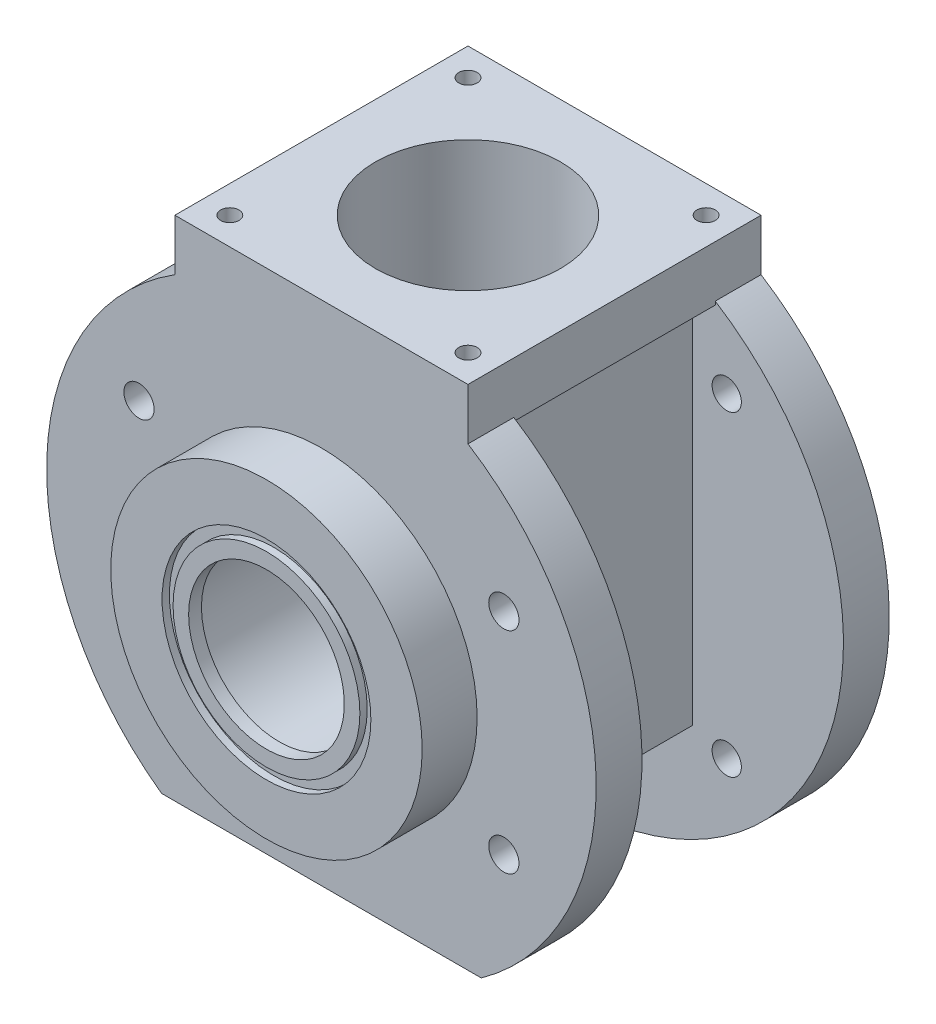
SolidWorks part; units mm, degrees
ref_plane "Front Plane" through (0, 0, 0) normal (0, 0, 1) x (1, 0, 0)
ref_plane "Top Plane" through (0, 0, 0) normal (0, 1, 0) x (1, 0, 0)
ref_plane "Right Plane" through (0, 0, 0) normal (1, 0, 0) x (0, 0, -1)
ref_plane "Plane1" through (0, 0, -520.693) normal (0, 0, -1) x (-1, 0, 0)
sketch "Sketch1" plane through (0, 0, -520.693) normal (0, 0, -1) x (-1, 0, 0)
  line L0 (-441.2306, 361.6297) -> (-601.2306, 361.6297)
  arc A0 (-601.2306, 361.6297) -> (-441.2306, 361.6297) centre (-521.2306, 234.744) ccw
  dimension "D1" = 150
  dimension "D2" = 80
extrude "Boss-Extrude1" add sketch "Sketch1" against normal blind 25
sketch "Sketch2" plane through (0, 0, -495.693) normal (0, 0, 1) x (1, 0, 0)
  line L0 (441.2306, 361.6297) -> (601.2306, 361.6297)
  line L1 (601.2306, 361.6297) -> (601.2306, 154.744)
  line L2 (601.2306, 154.744) -> (441.2306, 154.744)
  line L3 (441.2306, 154.744) -> (441.2306, 361.6297)
  dimension "D1" = 160
  dimension "D2" = 206.8858
extrude "Boss-Extrude2" add sketch "Sketch2" along normal blind 110
sketch "Sketch3" plane through (0, 0, -385.693) normal (0, 0, 1) x (1, 0, 0)
  line L0 (608.5003, 112.744) -> (433.9609, 112.744)
  line L1 (441.2306, 361.6297) -> (601.2306, 361.6297)
  line L2 (441.2306, 361.6297) -> (441.2306, 154.744) construction
  line L3 (441.2306, 154.744) -> (601.2306, 154.744) construction
  arc A0 (601.2306, 361.6297) -> (608.5003, 112.744) centre (521.2306, 234.744) cw
  arc A1 (433.9609, 112.744) -> (441.2306, 361.6297) centre (521.2306, 234.744) cw
  dimension "D1" = 150
  dimension "D2" = 150
  dimension "D3" = 80
  dimension "D4" = 160
  dimension "D5" = 167.2697
  dimension "D6" = 80
extrude "Boss-Extrude3" add sketch "Sketch3" along normal blind 25
sketch "Sketch4" plane through (0, 361.6297, 0) normal (0, 1, 0) x (-1, 0, 0)
  line L0 (-601.2306, -520.693) -> (-601.2306, -360.693)
  line L1 (-601.2306, -360.693) -> (-441.2306, -360.693)
  line L2 (-441.2306, -360.693) -> (-441.2306, -520.693)
  line L3 (-441.2306, -520.693) -> (-601.2306, -520.693)
  line L4 (-441.2306, -495.693) -> (-441.2306, -520.693) construction
  line L5 (-441.2306, -520.693) -> (-601.2306, -520.693) construction
  dimension "D1" = 160
  dimension "D2" = 160
extrude "Boss-Extrude4" add sketch "Sketch4" along normal blind 28.1142
ref_plane "Plane2" through (601.2306, 0, 0) normal (1, 0, 0) x (0, 0, -1)
ref_plane "Plane3" through (588.7306, 0, 0) normal (-1, 0, 0) x (0, -1, 0)
sketch "Sketch6" plane through (588.7306, 0, 0) normal (-1, 0, 0) x (0, -1, 0)
  line L0 (-359.744, -495.693) -> (-154.744, -495.693)
  line L1 (-154.744, -495.693) -> (-154.744, -385.693)
  line L2 (-154.744, -385.693) -> (-359.744, -385.693)
  line L3 (-359.744, -385.693) -> (-359.744, -495.693)
  dimension "D1" = 205
  dimension "D2" = 110
extrude "Cut-Extrude1" cut sketch "Sketch6" against normal up to surface up to plane "Plane2"
ref_plane "Plane4" through (0, 154.744, 0) normal (0, -1, 0) x (1, 0, 0)
ref_plane "Plane5" through (0, 359.744, 0) normal (0, 1, 0) x (1, 0, 0)
sketch "Sketch8" plane through (0, 359.744, 0) normal (0, 1, 0) x (1, 0, 0)
  line L0 (453.7306, 495.693) -> (441.2306, 495.693)
  line L1 (441.2306, 495.693) -> (441.2306, 385.693)
  line L2 (441.2306, 385.693) -> (453.7306, 385.693)
  line L3 (453.7306, 385.693) -> (453.7306, 495.693)
  dimension "D1" = 12.5
  dimension "D2" = 110
extrude "Cut-Extrude2" cut sketch "Sketch8" against normal up to surface up to plane "Plane4"
sketch "Sketch9" plane through (0, 0, -360.693) normal (0, 0, 1) x (1, 0, 0)
  line L0 (601.2306, 389.744) -> (601.2306, 361.6297) construction
  line L1 (441.2306, 389.744) -> (601.2306, 389.744) construction
  circle A0 centre (521.2306, 234.744) radius 85
  dimension "D1" = 170
  dimension "D2" = 80
  dimension "D3" = 155
extrude "Boss-Extrude5" add sketch "Sketch9" along normal blind 30
hole_wizard "Hole1" positions "Sketch11" profile "Sketch10" legacy
sketch "Sketch11" plane through (0, 0, -330.693) normal (0, 0, 1) x (1, 0, 0)
  point P0 (521.2306, 234.744)
sketch "Sketch10" plane through (521.2306, 234.744, -330.693) normal (1, 0, 0) x (0, -1, 0)
  line L0 (0, 0) -> (0, 4)
  line L1 (0, 4) -> (57, 4)
  line L2 (57, 4) -> (57, 0)
  line L3 (57, 0) -> (0, 0)
  line L4 (0, 110) -> (0, -10) construction
  dimension "直径" = 114
  dimension "深度" = 4
ref_plane "Plane6" through (0, 234.744, 0) normal (0, 1, 0) x (1, 0, 0)
sketch "Sketch12" plane through (0, 234.744, 0) normal (0, 1, 0) x (1, 0, 0)
  line L0 (631.2306, 528.693) -> (521.2306, 528.693)
  line L1 (521.2306, 528.693) -> (521.2306, 520.693)
  line L2 (521.2306, 520.693) -> (631.2306, 520.693)
  line L3 (631.2306, 520.693) -> (631.2306, 528.693)
  line L4 (521.2306, 528.693) -> (521.2306, 520.693) construction
  dimension "D1" = 110
  dimension "D2" = 8
revolve "Revolve1" add sketch "Sketch12" angle 360 about L4
sketch "Sketch13" plane through (0, 234.744, 0) normal (0, 1, 0) x (1, 0, 0)
  line L0 (572.2306, 334.693) -> (521.2306, 334.693)
  line L1 (521.2306, 334.693) -> (521.2306, 330.693)
  line L2 (521.2306, 330.693) -> (572.2306, 330.693)
  line L3 (572.2306, 330.693) -> (572.2306, 334.693)
  line L4 (521.2306, 334.693) -> (521.2306, 330.693) construction
  dimension "D1" = 51
  dimension "D2" = 4
revolve "Revolve2" add sketch "Sketch13" angle 360 about L4
hole_wizard "Ø16.0 (16) diameter hole1" positions "Sketch15" profile "Sketch14" hole size "Ø16.0" standard "ANSI Metric"
sketch "Sketch15" plane through (0, 0, -520.693) normal (0, 0, -1) x (-1, 0, 0)
  point P0 (-434.9636, 321.011)
  point P1 (-607.4977, 148.4769)
  point P2 (-434.9636, 148.4769)
  point P3 (-607.4977, 321.011)
sketch "Sketch14" plane through (434.9636, 321.011, -520.693) normal (1, 0, 0) x (0, 1, 0)
  line L0 (0, 0) -> (0, 25)
  line L1 (0, 25) -> (8, 25)
  line L2 (8, 25) -> (8, 0)
  line L5 (8, 0) -> (0, 0)
  line L11 (0, -6.35) -> (0, 107.95) construction
  dimension "通孔孔直径" = 16
  dimension "通孔孔深度" = 25
hole_wizard "Ø16.5 (16.5) diameter hole1" positions "Sketch17" profile "Sketch16" hole size "Ø16.5" standard "ANSI Metric"
sketch "Sketch17" plane through (0, 0, -385.693) normal (0, 0, -1) x (-1, 0, 0)
  point P0 (-620.8236, 292.244)
  point P1 (-421.6377, 177.244)
  point P2 (-421.6377, 292.244)
  point P3 (-620.8236, 177.244)
sketch "Sketch16" plane through (620.8236, 292.244, -385.693) normal (1, 0, 0) x (0, 1, 0)
  line L0 (0, 0) -> (0, 55)
  line L1 (0, 55) -> (8.25, 55)
  line L2 (8.25, 55) -> (8.25, 0)
  line L5 (8.25, 0) -> (0, 0)
  line L11 (0, -6.35) -> (0, 107.95) construction
  dimension "通孔孔直径" = 16.5
  dimension "通孔孔深度" = 55
hole_wizard "Ø10.0 (10) diameter hole1" positions "Sketch19" profile "Sketch18" hole size "Ø10.0" standard "ANSI Metric"
sketch "Sketch19" plane through (0, 389.744, 0) normal (0, 1, 0) x (1, 0, 0)
  point P0 (456.2306, 505.693)
  point P1 (586.2306, 505.693)
  point P2 (586.2306, 375.693)
  point P3 (456.2306, 375.693)
sketch "Sketch18" plane through (456.2306, 389.744, -505.693) normal (1, 0, 0) x (0, 0, 1)
  line L0 (0, 0) -> (0, 30)
  line L1 (0, 30) -> (5, 30)
  line L2 (5, 30) -> (5, 0)
  line L5 (5, 0) -> (0, 0)
  line L10 (0, 30) -> (-5, 30) construction
  line L11 (0, -6.35) -> (0, 107.95) construction
  dimension "孔直径" = 10
  dimension "孔深度" = 30
  dimension "导头角度" = 180
hole_wizard "Ø8.0 (8) diameter hole1" positions "Sketch21" profile "Sketch20" hole size "Ø8.0" standard "ANSI Metric"
sketch "Sketch21" plane through (0, 154.744, 0) normal (0, -1, 0) x (-1, 0, 0)
  point P0 (-468.7306, 480.693)
  point P1 (-573.7306, 400.693)
  point P2 (-573.7306, 480.693)
  point P3 (-468.7306, 400.693)
sketch "Sketch20" plane through (468.7306, 154.744, -480.693) normal (1, 0, 0) x (0, 0, -1)
  line L0 (0, 0) -> (0, 18)
  line L1 (0, 18) -> (4, 18)
  line L2 (4, 18) -> (4, 0)
  line L5 (4, 0) -> (0, 0)
  line L10 (0, 18) -> (-4, 18) construction
  line L11 (0, -6.35) -> (0, 107.95) construction
  dimension "孔直径" = 8
  dimension "孔深度" = 18
  dimension "导头角度" = 180
hole_wizard "M52 clearance hole1" positions "Sketch23" profile "Sketch22" hole size "M52" standard "ANSI Metric"
sketch "Sketch23" plane through (0, 154.744, 0) normal (0, -1, 0) x (-1, 0, 0)
  point P0 (-521.2306, 440.693)
sketch "Sketch22" plane through (521.2306, 154.744, -440.693) normal (1, 0, 0) x (0, 0, -1)
  line L0 (0, 0) -> (0, 40)
  line L1 (0, 40) -> (30, 40)
  line L2 (30, 40) -> (30, 0)
  line L5 (30, 0) -> (0, 0)
  line L10 (0, 40) -> (-30, 40) construction
  line L11 (0, -6.35) -> (0, 107.95) construction
  dimension "孔直径" = 60
  dimension "孔深度" = 40
  dimension "导头角度" = 180
hole_wizard "M90 clearance hole1" positions "Sketch25" profile "Sketch24" hole size "M90" standard "ANSI Metric"
sketch "Sketch25" plane through (0, 389.744, 0) normal (0, 1, 0) x (1, 0, 0)
  point P0 (521.2306, 440.693)
sketch "Sketch24" plane through (521.2306, 389.744, -440.693) normal (1, 0, 0) x (0, 0, 1)
  line L0 (0, 0) -> (0, 155)
  line L1 (0, 155) -> (50.5, 155)
  line L2 (50.5, 155) -> (50.5, 0)
  line L5 (50.5, 0) -> (0, 0)
  line L10 (0, 155) -> (-50.5, 155) construction
  line L11 (0, -6.35) -> (0, 107.95) construction
  dimension "孔直径" = 101
  dimension "孔深度" = 155
  dimension "导头角度" = 180
hole_wizard "M80 counterbore hole1" positions "Sketch27" profile "Sketch26" counterbore size "M80" standard "ANSI Metric"
sketch "Sketch27" plane through (0, 0, -528.693) normal (0, 0, -1) x (-1, 0, 0)
  point P0 (-521.2306, 234.744)
sketch "Sketch26" plane through (521.2306, 234.744, -528.693) normal (1, 0, 0) x (0, 1, 0)
  line L0 (0, 0) -> (0, 198)
  line L1 (0, 198) -> (42.5, 198)
  line L3 (42.5, 198) -> (42.5, 191)
  line L4 (42.5, 191) -> (49.5, 191)
  line L5 (49.5, 191) -> (49.5, 0)
  line L7 (49.5, 0) -> (0, 0)
  line L11 (0, -6.35) -> (0, 107.95) construction
  dimension "通孔孔直径" = 85
  dimension "通孔孔深度" = 198
  dimension "柱形沉头孔直径" = 99
  dimension "柱形沉头孔深度" = 191
